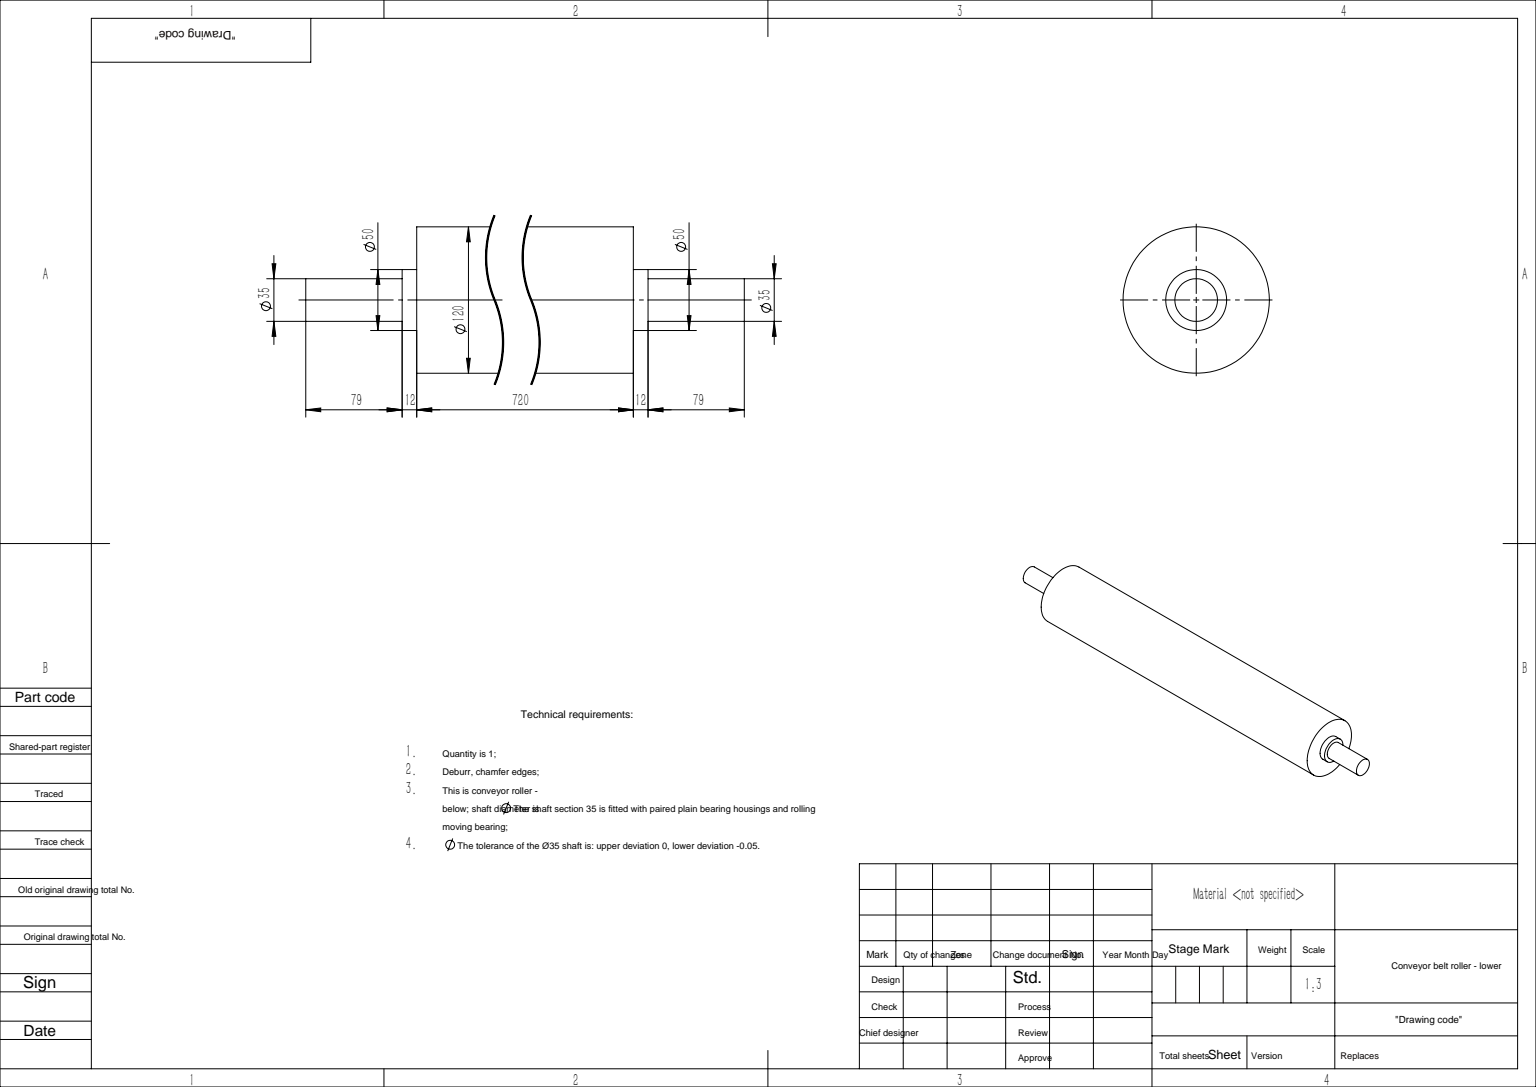
SolidWorks part; units mm, degrees
ref_plane "前视基准面" through (0, 0, 0) normal (0, 0, 1) x (1, 0, 0)
ref_plane "上视基准面" through (0, 0, 0) normal (0, 1, 0) x (1, 0, 0)
ref_plane "右视基准面" through (0, 0, 0) normal (1, 0, 0) x (0, 0, -1)
sketch "草图1" plane through (0, 0, 0) normal (0, 0, 1) x (1, 0, 0)
  line L0 (0, 0) -> (82.8035, 0) construction
  line L1 (0, 0) -> (0, 35.4694) construction
  line L2 (-360, 60) -> (360, 60)
  line L3 (360, 60) -> (360, 25)
  line L4 (360, 25) -> (372, 25)
  line L5 (372, 25) -> (372, 17.5)
  line L6 (372, 17.5) -> (451, 17.5)
  line L7 (451, 17.5) -> (451, 0)
  line L8 (-451, 17.5) -> (-451, 0)
  line L9 (-372, 17.5) -> (-451, 17.5)
  line L10 (-372, 25) -> (-372, 17.5)
  line L11 (-360, 25) -> (-372, 25)
  line L12 (-360, 60) -> (-360, 25)
  line L13 (-451, 0) -> (451, 0)
  point P17 (0, 60)
  dimension "D1" = 60
  dimension "D2" = 360
  dimension "D3" = 12
  dimension "D4" = 25
  dimension "D5" = 17.5
  dimension "D6" = 79
revolve "旋转1" add sketch "草图1" angle 360 about L13
